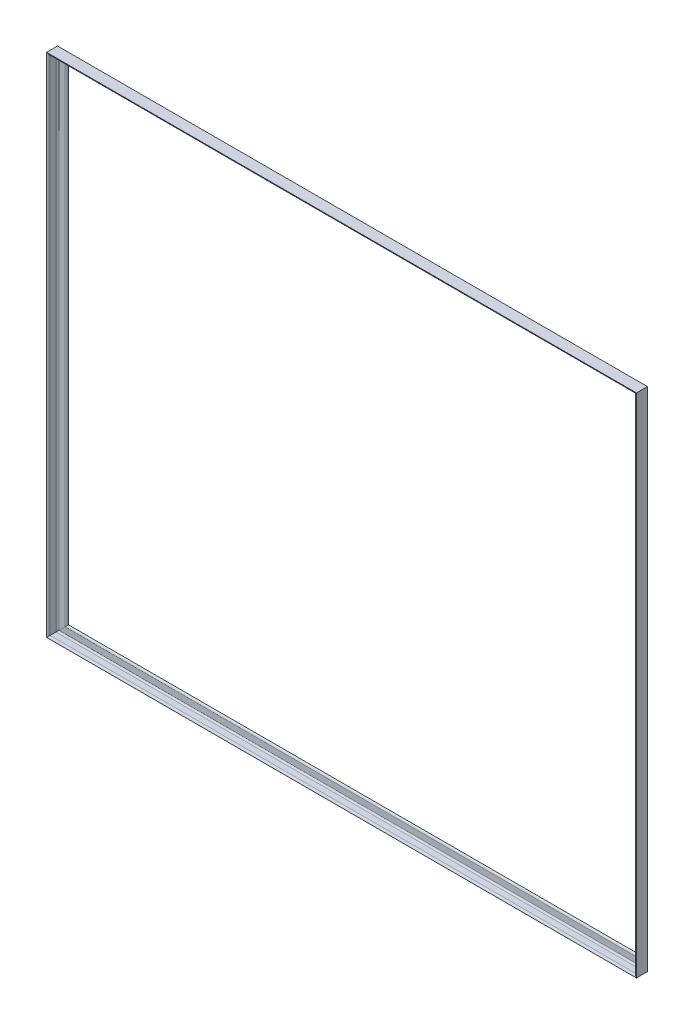
SolidWorks part; units mm, degrees
ref_plane "Front Plane" through (0, 0, 0) normal (0, 0, 1) x (1, 0, 0)
ref_plane "Top Plane" through (0, 0, 0) normal (0, 1, 0) x (1, 0, 0)
ref_plane "Right Plane" through (0, 0, 0) normal (1, 0, 0) x (0, 0, -1)
sketch "草图1" plane through (0, 0, 0) normal (0, 0, 1) x (1, 0, 0)
  line L1 (-674, 579) -> (674, 579)
  line L2 (-674, 579) -> (-674, -579)
  line L3 (-674, -579) -> (674, -579)
  line L4 (674, 579) -> (674, -579)
  line L5 (-674, 579) -> (674, -579) construction
  line L6 (-674, -579) -> (674, 579) construction
  point P0 (0, 0)
  dimension "D1" = 1348
  dimension "D2" = 1158
other "Angle iron - configured 25 X 25 X 4(1)"
ref_plane "Plane2" through (-674, 579, 0) normal (0, -1, 0) x (1, 0, 0)
sketch "Sketch1" plane through (-674, 579, 0) normal (0, -1, 0) x (1, 0, 0)
  line L0 (0, 0) -> (0, 25)
  line L1 (0, 12.5) -> (4, 12.5) construction
  line L2 (4, 21) -> (4, 7.5)
  line L3 (7.5, 4) -> (21, 4)
  line L4 (12.5, 4) -> (12.5, 0) construction
  line L5 (25, 0) -> (0, 0)
  arc A0 (25, 0) -> (21, 4) centre (21, 0) ccw
  arc A1 (0, 25) -> (4, 21) centre (0, 21) cw
  arc A2 (7.5, 4) -> (4, 7.5) centre (7.5, 7.5) cw
  point P10 (12.5, 0)
  point P14 (0, 12.5)
  point P15 (4, 12.5)
  point P16 (12.5, 4)
  point P17 (4, 25)
  point P18 (25, 4)
  point P21 (0, 0)
  dimension "D2" = 4
  dimension "D3" = 25
  dimension "Radius_1" = 3.5
  dimension "D1" = 4
